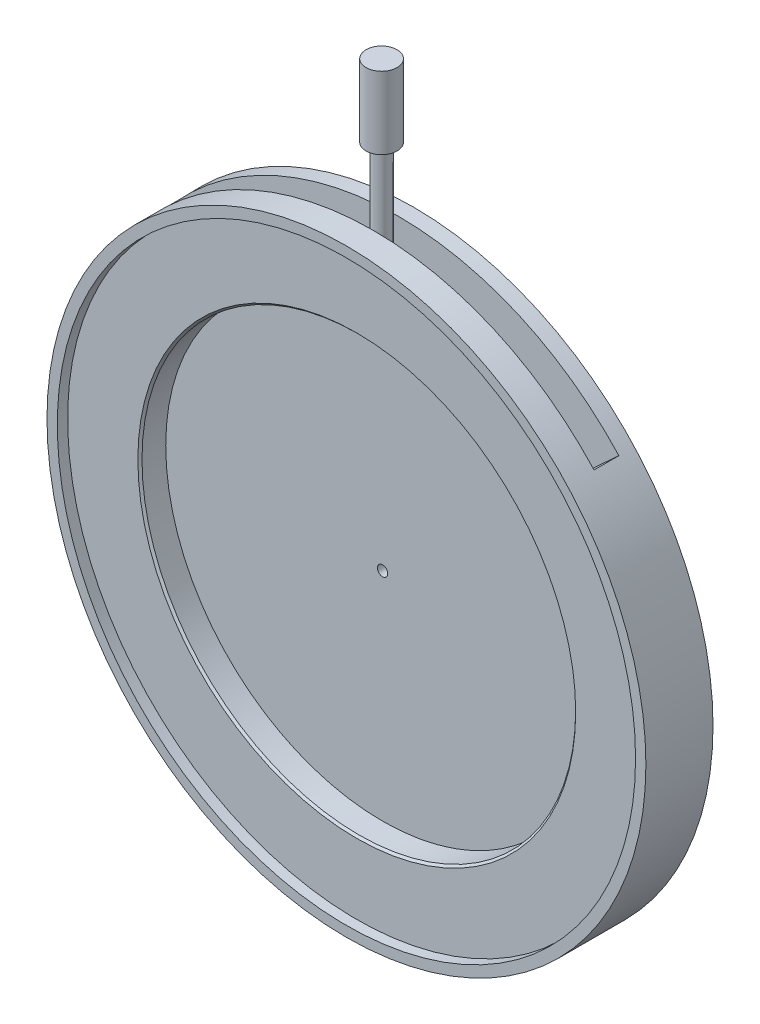
SolidWorks part; units mm, degrees
material "6061-T6 (SS)"
ref_plane "前视基准面" through (0, 0, 0) normal (0, 0, 1) x (1, 0, 0)
ref_plane "上视基准面" through (0, 0, 0) normal (0, 1, 0) x (1, 0, 0)
ref_plane "右视基准面" through (0, 0, 0) normal (1, 0, 0) x (0, 0, -1)
sketch "草图1" plane through (0, 0, 0) normal (0, 0, 1) x (1, 0, 0)
  circle A0 centre (0, 0) radius 29
  circle A1 centre (0, 0) radius 21
  dimension "D1" = 58
  dimension "D2" = 42
extrude "凸台-拉伸1" add sketch "草图1" along normal blind 6.5
sketch "草图7" plane through (0, 0, 6.5) normal (0, 0, 1) x (1, 0, 0)
  circle A0 centre (0, 0) radius 28
  dimension "D1" = 56
extrude "切除-拉伸5" cut sketch "草图7" against normal blind 1
sketch "草图9" plane through (0, 0, 0) normal (0, 0, -1) x (-1, 0, 0)
  line L0 (0, 0) -> (0, 32.7234) construction
  line L1 (-18.4319, 16.8898) -> (-21.381, 19.5921)
  line L2 (18.4319, 16.8898) -> (21.381, 19.5921)
  arc A0 (18.4319, 16.8898) -> (-18.4319, 16.8898) centre (0, 0) ccw
  arc A1 (21.381, 19.5921) -> (-21.381, 19.5921) centre (0, 0) ccw
  circle A2 centre (0, 0) radius 29 construction
  dimension "D2" = 50
  dimension "D1" = 95
extrude "切除-拉伸6" cut sketch "草图9" against normal blind 2.4 from offset 1.5 offset against normal yes
sketch "草图10" plane through (0, 0, 0) normal (1, 0, 0) x (0, 0, -1)
  line L0 (-3.9, 29) -> (-2.2934, 29) construction
  line L1 (-3.0967, 29) -> (-3.0967, 43) construction
  line L2 (-3.0967, 43) -> (-1.5967, 43)
  line L3 (-1.5967, 43) -> (-1.5967, 36)
  line L4 (-1.5967, 36) -> (-2.2967, 36)
  line L5 (-2.2967, 36) -> (-2.2967, 29)
  line L6 (-2.2967, 29) -> (-3.0967, 29)
  line L7 (-3.0967, 29) -> (-3.0967, 43)
  point P8 (0, 0)
  point P9 (0, 0)
  point P10 (0, 0)
  point P11 (0, 0)
  dimension "D1" = 3
  dimension "D2" = 14
  dimension "D3" = 7
  dimension "D4" = 0.8
revolve "旋转4" add sketch "草图10" angle 360 about L7
other "移动面1" face at (0, 29, 2.2967) parameters "D1"=5
sketch "草图11" plane through (0, 0, 6.5) normal (0, 0, 1) x (1, 0, 0)
  circle A0 centre (0, 0) radius 22.5
  circle A2 centre (0, 0) radius 0.5
  dimension "D1" = 45
  dimension "D2" = 1
extrude "凸台-拉伸2" add sketch "草图11" against normal blind 1 from offset 3.5 separate body offset against normal yes
chamfer "倒角1" distance 0.2 angle 45 1 edges at (21, 0, 5.5)
